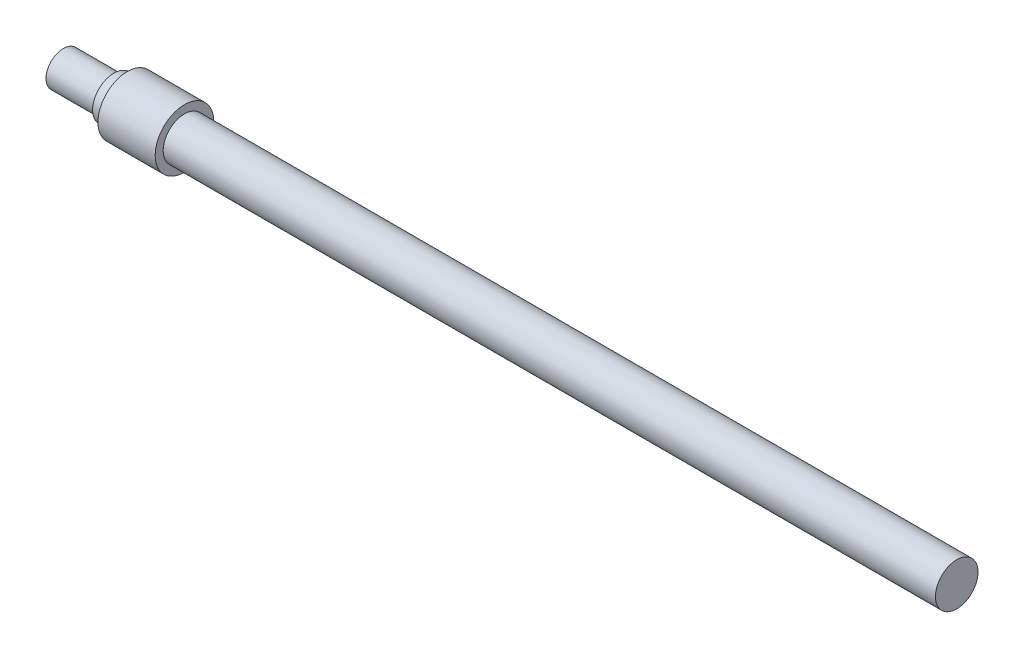
SolidWorks part; units mm, degrees
ref_plane "前视基准面" through (0, 0, 0) normal (0, 0, 1) x (1, 0, 0)
ref_plane "上视基准面" through (0, 0, 0) normal (0, 1, 0) x (1, 0, 0)
ref_plane "右视基准面" through (0, 0, 0) normal (1, 0, 0) x (0, 0, -1)
other "Configuration Table"
sketch "草图1" plane through (0, 0, 0) normal (0, 0, 1) x (1, 0, 0)
  line L0 (-119.5804, 0) -> (506.9653, 0) construction
  line L1 (-108.8246, 0) -> (-108.8246, 13)
  line L2 (-108.8246, 13) -> (-70.8246, 13)
  line L3 (-70.8246, 13) -> (-70.8246, 16)
  line L4 (-70.8246, 16) -> (-60.8246, 16)
  line L5 (-60.8246, 16) -> (-60.8246, 22)
  line L6 (-60.8246, 22) -> (-17.8246, 22)
  line L7 (-17.8246, 22) -> (-17.8246, 16)
  line L8 (562.1754, 16) -> (562.1754, 0)
  line L9 (-17.8246, 16) -> (562.1754, 16)
  line L10 (-108.8246, 0) -> (562.1754, 0)
  dimension "D1" = 16
  dimension "D2" = 38
  dimension "D3" = 10
  dimension "D4" = 580
revolve "旋转1" add sketch "草图1" angle 360 about L0
